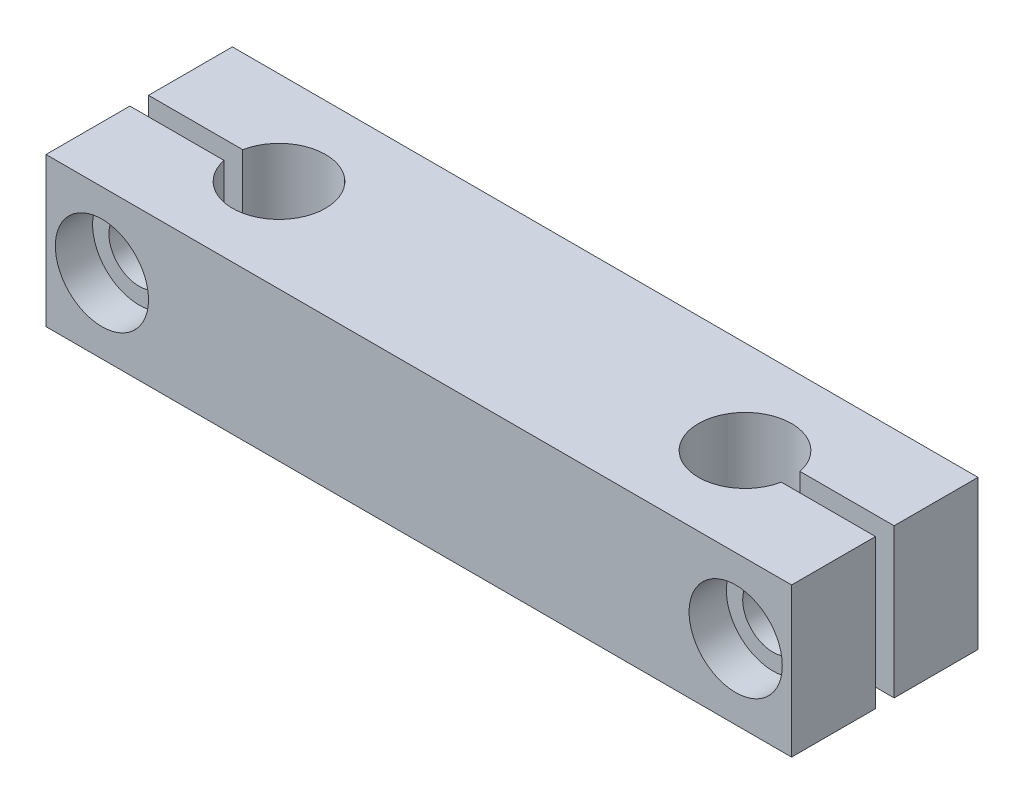
from build123d import *

# Parameters (mm, degrees)
SKETCH1_W                  = 80
SKETCH1_H                  = 16
BOSS_EXTRUDE1_DEPTH        = 20
SKETCH2_R                  = 5
CUT_EXTRUDE1_DEPTH         = 20
SKETCH3_W                  = 12.438334811
SKETCH3_H                  = 2
CUT_EXTRUDE2_DEPTH         = 30
M6_TAPPED_HOLE1_AT_2_COUNT = 2
M6_TAPPED_HOLE1_AT_2_PITCH = 68
SKETCH7_R                  = 3.25
CUT_EXTRUDE3_DEPTH         = 30
SKETCH8_R                  = 5
CUT_EXTRUDE7_DEPTH         = 4


with BuildPart() as part:
    # Sketch1 → Boss-Extrude1 (new body)
    with BuildSketch(Plane.XY):
        with Locations((-40, 8)):
            Rectangle(SKETCH1_W, SKETCH1_H)
    extrude(amount=BOSS_EXTRUDE1_DEPTH)

    # Sketch2 → Cut-Extrude1 (cut)
    with BuildSketch(Plane.XZ):
        with Locations((-15, 10)):
            Circle(SKETCH2_R)
        with Locations((-65, 10)):
            Circle(SKETCH2_R)
    extrude(amount=-CUT_EXTRUDE1_DEPTH, mode=Mode.SUBTRACT)

    # Sketch3 → Cut-Extrude2 (cut)
    with BuildSketch(Plane.XZ):
        with Locations((-4.725841747, 10)):
            Rectangle(SKETCH3_W, SKETCH3_H)
        with Locations((-75.274158254, 10)):
            Rectangle(SKETCH3_W, SKETCH3_H)
    extrude(amount=-CUT_EXTRUDE2_DEPTH, mode=Mode.SUBTRACT)

    # Sketch4 → M6 Tapped Hole1 (revolve, cut)
    with BuildSketch(Plane(origin=(-6, 8, 9), x_dir=(0, -1, 0), z_dir=(1, 0, 0))):
        Polygon((0, 0), (0, 18.502151548), (2.5, 17), (2.5, 0), align=None)
    m6_tapped_hole1 = revolve(axis=Axis((-6, 8, 15.35), (0, 0, -1)), mode=Mode.SUBTRACT)

    # M6 Tapped Hole1 at 2: M6 Tapped Hole1 ×2
    with Locations(*[(-i * M6_TAPPED_HOLE1_AT_2_PITCH, 0, 0) for i in range(1, M6_TAPPED_HOLE1_AT_2_COUNT)]):
        add(m6_tapped_hole1, mode=Mode.SUBTRACT)

    # Sketch7 → Cut-Extrude3 (cut)
    with BuildSketch(Plane(origin=(0, 0, 11), x_dir=(-1, 0, 0), z_dir=(0, 0, -1))):
        with Locations((74, 8)):
            Circle(SKETCH7_R)
        with Locations((6, 8)):
            Circle(SKETCH7_R)
    extrude(amount=-CUT_EXTRUDE3_DEPTH, mode=Mode.SUBTRACT)

    # Sketch8 → Cut-Extrude7 (cut)
    with BuildSketch(Plane.XY.offset(20)):
        with Locations((-6, 8)):
            Circle(SKETCH8_R)
        with Locations((-74, 8)):
            Circle(SKETCH8_R)
    extrude(amount=-CUT_EXTRUDE7_DEPTH, mode=Mode.SUBTRACT)


solid = part.part
